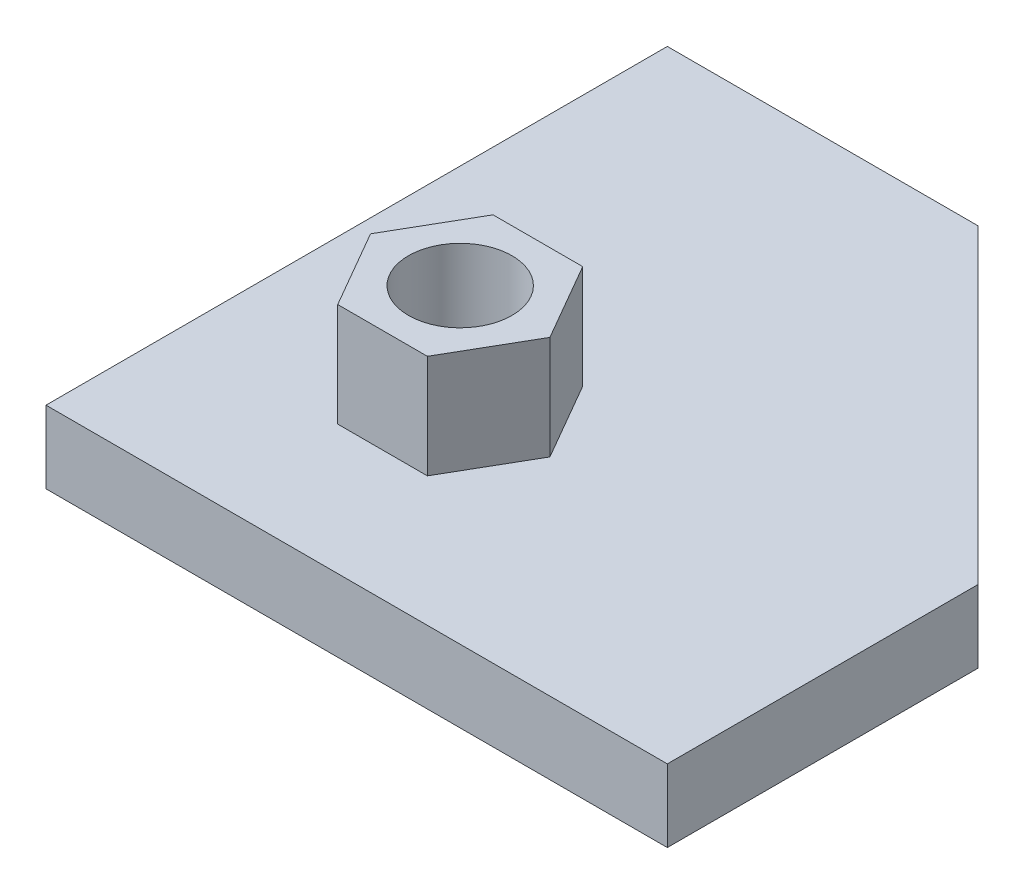
SolidWorks part; units mm, degrees
material "Q235"
ref_plane "Front Plane" through (0, 0, 0) normal (0, 0, 1) x (1, 0, 0)
ref_plane "Top Plane" through (0, 0, 0) normal (0, 1, 0) x (1, 0, 0)
ref_plane "Right Plane" through (0, 0, 0) normal (1, 0, 0) x (0, 0, -1)
sketch "Sketch2" plane through (0, 0, 0) normal (0, 1, 0) x (1, 0, 0)
  line L0 (0, 0) -> (0, 120)
  line L1 (0, 120) -> (60, 120)
  line L2 (60, 120) -> (120, 60)
  line L3 (120, 60) -> (120, 0)
  line L4 (120, 0) -> (0, 0)
  dimension "D1" = 120
  dimension "D2" = 120
  dimension "D3" = 60
  dimension "D4" = 60
extrude "Boss-Extrude1" add sketch "Sketch2" along normal blind 14
sketch "Sketch3" plane through (0, 14, 0) normal (0, 1, 0) x (1, 0, 0)
  line L0 (40, 0) -> (40, 40) construction
  line L1 (0, 0) -> (120, 0) construction
  line L2 (40, 40) -> (0, 40) construction
  line L3 (0, 120) -> (0, 0) construction
  circle A0 centre (40, 40) radius 11.5
  dimension "D1" = 40
  dimension "D3" = 23
  dimension "D2" = 40
extrude "Cut-Extrude1" cut sketch "Sketch3" against normal blind 14
sketch "Sketch4" plane through (0, 14, 0) normal (0, 1, 0) x (1, 0, 0)
  line L1 (57.3205, 40) -> (48.6603, 55)
  line L2 (48.6603, 55) -> (31.3397, 55)
  line L3 (31.3397, 55) -> (22.6795, 40)
  line L4 (22.6795, 40) -> (31.3397, 25)
  line L5 (31.3397, 25) -> (48.6603, 25)
  line L6 (48.6603, 25) -> (57.3205, 40)
  circle A1 centre (40, 40) radius 15 construction
  circle A2 centre (40, 40) radius 10
  dimension "D1" = 20
  dimension "D2" = 30
extrude "Boss-Extrude2" add sketch "Sketch4" along normal blind 20
